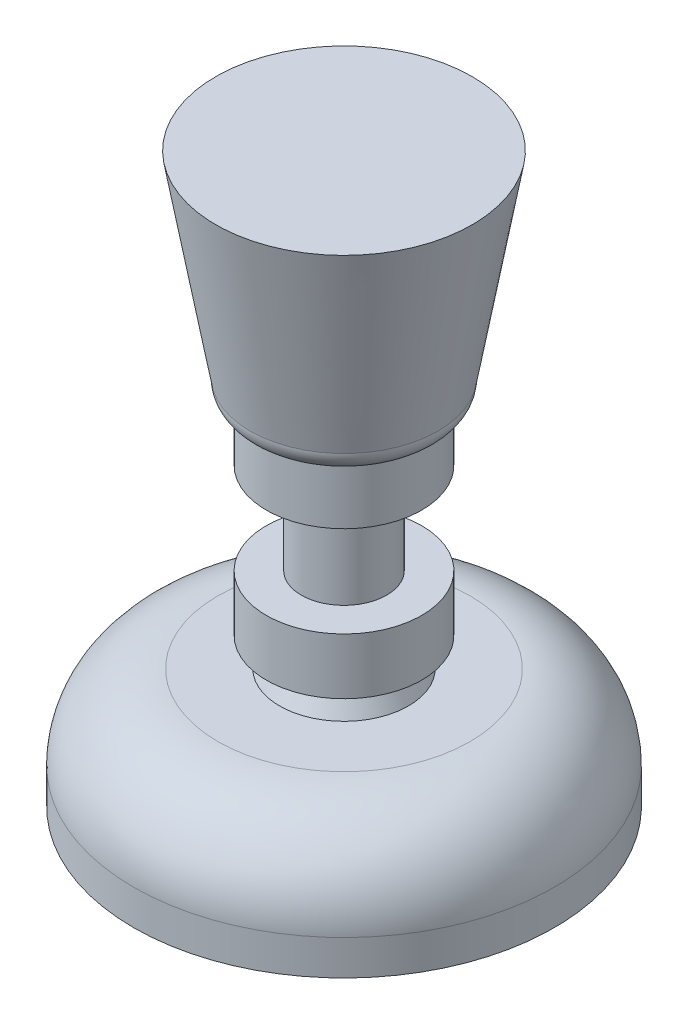
SolidWorks part; units mm, degrees
ref_plane "前视基准面" through (0, 0, 0) normal (0, 0, 1) x (1, 0, 0)
ref_plane "上视基准面" through (0, 0, 0) normal (0, 1, 0) x (1, 0, 0)
ref_plane "右视基准面" through (0, 0, 0) normal (1, 0, 0) x (0, 0, -1)
sketch "草图1" plane through (0, 0, 0) normal (0, 0, 1) x (1, 0, 0)
  line L0 (0, 0) -> (0, 11562.632) construction
  line L1 (0, -19.5161) -> (24, -19.5161)
  line L2 (24, -19.5161) -> (24, -16.5161)
  line L3 (24, -16.5161) -> (30, -16.5161)
  line L4 (30, -16.5161) -> (30, -11.5161)
  line L7 (18, 0.4839) -> (9.2, 0.4839)
  line L8 (9.2, 0.4839) -> (8.0896, 2.6115)
  line L9 (8.0896, 2.6115) -> (8.0896, 4.6115)
  line L10 (8.0896, 4.6115) -> (11.0896, 4.6115)
  line L11 (11.0896, 4.6115) -> (11.0896, 12.6115)
  line L12 (11.0896, 12.6115) -> (6.0896, 12.6115)
  line L13 (6.0896, 12.6115) -> (6.0896, 25.6115)
  line L14 (6.0896, 25.6115) -> (11.0896, 25.6115)
  line L15 (11.0896, 25.6115) -> (11.0896, 33.6115)
  line L16 (0, 64.4839) -> (18.3, 64.4839)
  line L17 (18.3, 64.4839) -> (13.3996, 36.5311)
  line L18 (0, -19.5161) -> (0, 64.4839)
  arc A0 (30, -11.5161) -> (18, 0.4839) centre (18, -11.5161) ccw
  arc A3 (11.0896, 33.6115) -> (13.3996, 36.5311) centre (10.3996, 36.5311) ccw
  dimension "D18" = 6
  dimension "D1" = 24
  dimension "D2" = 3
  dimension "D3" = 6
  dimension "D4" = 5
  dimension "D5" = 8
  dimension "D6" = 12
  dimension "D7" = 8.8
  dimension "D8" = 2.4
  dimension "D9" = 2
  dimension "D10" = 5
  dimension "D11" = 13
  dimension "D12" = 3
  dimension "D13" = 5
  dimension "D14" = 8
  dimension "D15" = 84
  dimension "D16" = 18.3
revolve "旋转1" add sketch "草图1" angle 360 about L0
